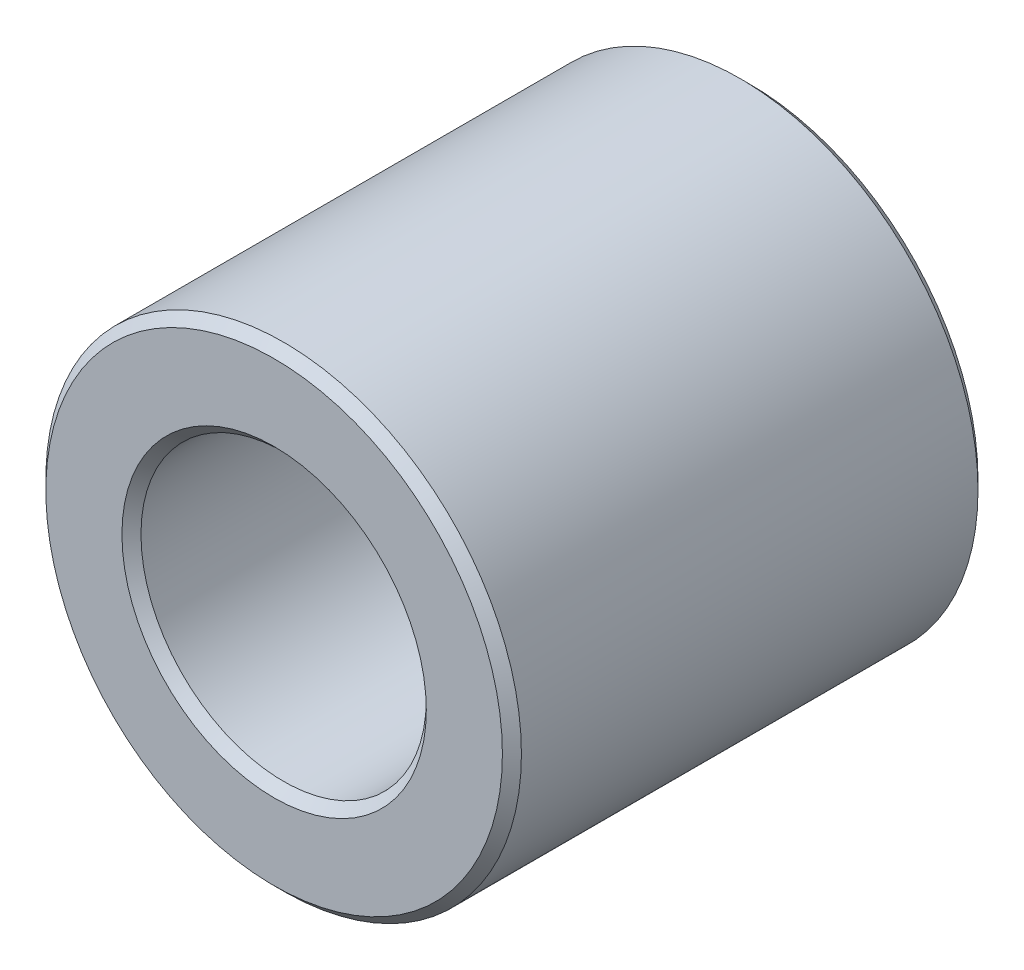
SolidWorks part; units mm, degrees
material "45#"
ref_plane "Front Plane" through (0, 0, 0) normal (0, 0, 1) x (1, 0, 0)
ref_plane "Top Plane" through (0, 0, 0) normal (0, 1, 0) x (1, 0, 0)
ref_plane "Right Plane" through (0, 0, 0) normal (1, 0, 0) x (0, 0, -1)
sketch "Sketch1" plane through (0, 0, 0) normal (0, 0, 1) x (1, 0, 0)
  circle A0 centre (0, 0) radius 25
  circle A1 centre (0, 0) radius 15
  dimension "D1" = 50
  dimension "D2" = 30
extrude "Boss-Extrude1" add sketch "Sketch1" along normal blind 50
chamfer "Chamfer1" distance 1 angle 45 4 edges at (15, 0, 0) (25, 0, 0) (15, 0, 50) (25, 0, 50)
